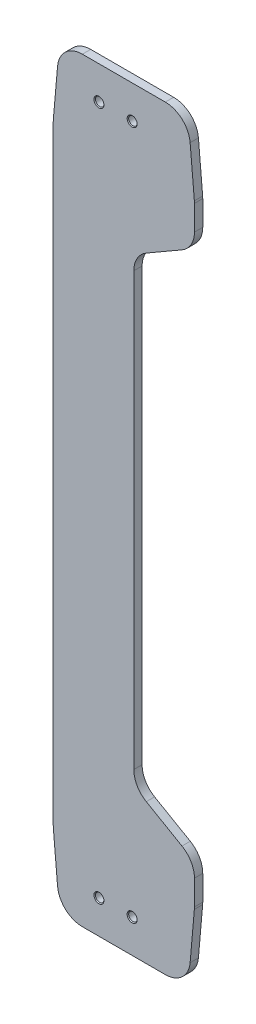
from build123d import *

# Parameters (mm, degrees)
EXTRUDE_1_DEPTH               = 10
HOLE_WIZARD_M12_1_D           = 10.2
HOLE_WIZARD_M12_1_CSINK_D     = 12.05
HOLE_WIZARD_M12_1_CSINK_ANGLE = 90


with BuildPart() as part:
    # 草图1 → 凸台-拉伸1 (new body)
    with BuildSketch(Plane.XY):
        with BuildLine():
            Line((-84.801934074, -1426.511579499), (-89.885840943, -1368.402258085))
            ThreePointArc((-89.885840943, -1368.402258085), (-89.971446647, -1367.096167423), (-90, -1365.787585802))
            Line((-90, -1365.787585802), (-90, -632.212414198))
            ThreePointArc((-90, -632.212414198), (-89.971446647, -630.903832577), (-89.885840943, -629.597741915))
            Line((-89.885840943, -629.597741915), (-84.801934074, -571.488420501))
            ThreePointArc((-84.801934074, -571.488420501), (-75.18379936, -551.984772679), (-54.916093131, -544.103092784))
            Line((-54.916093131, -544.103092784), (44.916093131, -544.103092784))
            ThreePointArc((44.916093131, -544.103092784), (65.18379936, -551.984772679), (74.801934074, -571.488420501))
            Line((74.801934074, -571.488420501), (79.885840943, -629.597741915))
            ThreePointArc((79.885840943, -629.597741915), (79.971446647, -630.903832577), (80, -632.212414198))
            Line((80, -632.212414198), (80, -662.212414198))
            ThreePointArc((80, -662.212414198), (75.980762114, -677.212414198), (65, -688.193176311))
            Line((65, -688.193176311), (22, -713.019237886))
            ThreePointArc((22, -713.019237886), (11.019237886, -724), (7, -739))
            Line((7, -739), (7, -1259))
            ThreePointArc((7, -1259), (11.019237886, -1274), (22, -1284.980762114))
            Line((22, -1284.980762114), (65, -1309.806823689))
            ThreePointArc((65, -1309.806823689), (75.980762114, -1320.787585802), (80, -1335.787585802))
            Line((80, -1335.787585802), (80, -1365.787585802))
            ThreePointArc((80, -1365.787585802), (79.971446647, -1367.096167423), (79.885840943, -1368.402258085))
            Line((79.885840943, -1368.402258085), (74.801934074, -1426.511579499))
            ThreePointArc((74.801934074, -1426.511579499), (65.18379936, -1446.015227321), (44.916093131, -1453.896907216))
            Line((44.916093131, -1453.896907216), (-54.916093131, -1453.896907216))
            ThreePointArc((-54.916093131, -1453.896907216), (-75.18379936, -1446.015227321), (-84.801934074, -1426.511579499))
        make_face()
    extrude(amount=EXTRUDE_1_DEPTH)

    # M12 螺纹孔1 (through all)
    with Locations(Plane(origin=(5, -1413.896907216, 10), x_dir=(1, 0, 0), z_dir=(0, 0, 1))):
        with Locations((0, 0), (-40, 0), (-40, 829.793814432), (0, 829.793814432)):
            CounterSinkHole(HOLE_WIZARD_M12_1_D / 2, HOLE_WIZARD_M12_1_CSINK_D / 2, counter_sink_angle=HOLE_WIZARD_M12_1_CSINK_ANGLE)


solid = part.part
